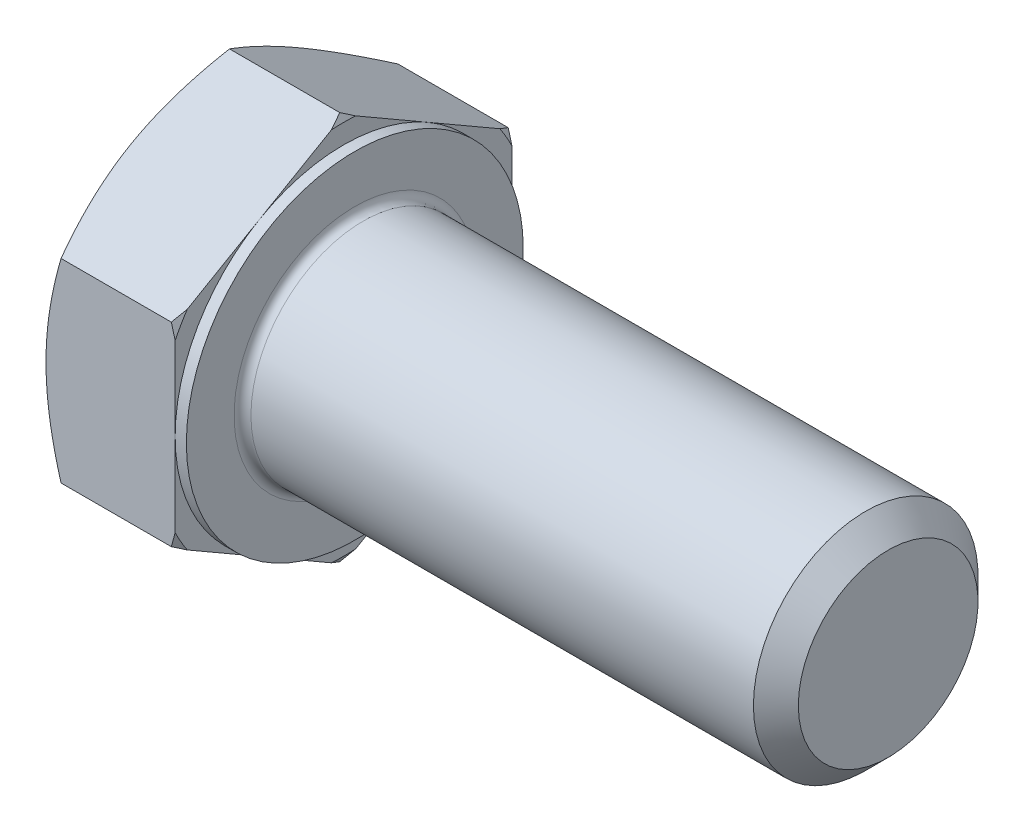
SolidWorks part; units mm, degrees
material "SAE2"
ref_plane "Front" through (0, 0, 0) normal (0, 0, 1) x (1, 0, 0)
ref_plane "Top" through (0, 0, 0) normal (0, 1, 0) x (1, 0, 0)
ref_plane "Right" through (0, 0, 0) normal (1, 0, 0) x (0, 0, -1)
sketch "Sketch1" plane through (0, 0, 0) normal (1, 0, 0) x (0, 0, -1)
  line L0 (12, 6.9282) -> (12, -6.9282)
  line L1 (-12, 6.9282) -> (-12, -6.9282)
  line L2 (12, -6.9282) -> (0, -13.8564)
  line L3 (0, -13.8564) -> (-12, -6.9282)
  line L4 (12, 6.9282) -> (0, 13.8564)
  line L5 (0, 13.8564) -> (-12, 6.9282)
  dimension "s" = 24
  dimension "D2" = 120
  dimension "D3" = 12
  dimension "D4" = 12
  dimension "D5" = 12
extrude "Base-Extrude" add sketch "Sketch1" along normal blind 10
sketch "Sketch2" plane through (0, 0, 0) normal (0, 0, 1) x (1, 0, 0)
  line L0 (0, 6.9282) -> (0, -6.9282) construction
  line L1 (0, 0) -> (48, 0)
  line L2 (0, 0) -> (0, 8)
  line L3 (0, 8) -> (27.8072, 8)
  line L4 (48, 0) -> (48, 6.268)
  line L5 (10, 13.8564) -> (10, 6.9282) construction
  line L7 (0, 0) -> (96.52, 0) construction
  line L8 (48, -6.268) -> (27.8072, -8) construction
  line L9 (0, -8) -> (27.8072, -8) construction
  line L10 (12, 15.24) -> (12, -1.27) construction
  line L11 (10, 15.24) -> (10, -1.27) construction
  line L12 (10, 6.9282) -> (10, -6.9282) construction
  line L13 (27.8072, 8) -> (48, 8)
  line L14 (48, 8) -> (48, 6.268)
  dimension "l" = 38
  dimension "m" = 16
  dimension "Minor_dia" = 12.536
  dimension "p" = 2
  dimension "h" = 38
revolve "Boss-Revolve1" add sketch "Sketch2" angle 360 about L7
cosmetic thread "Helix1" parameters "Thread_length"=36, "Thread_minor"=12.536
sketch "Sketch3" plane through (0, 0, 0) normal (0, 0, 1) x (1, 0, 0)
  line L0 (0, 12) -> (3.9585, 18.8564)
  line L1 (0, 13.8564) -> (0, 6.9282) construction
  line L2 (3.9585, 18.8564) -> (3.9585, 23.8564)
  line L3 (3.9585, 23.8564) -> (-10, 23.8564)
  line L4 (-10, 23.8564) -> (-10, 12)
  line L5 (-10, 12) -> (0, 12)
  line L6 (0, 0) -> (99.06, 0) construction
  line L7 (10, 13.8564) -> (0, 13.8564) construction
  dimension "D1" = 12
  dimension "D2" = 5
  dimension "D3" = 10
  dimension "D4" = 5
  dimension "Head_ch_ang" = 30
revolve "Cut-Revolve1" cut sketch "Sketch3" angle 360 about L6
sketch "Sketch5" plane through (0, 0, 0) normal (0, 0, 1) x (1, 0, 0)
  line L0 (10, 12) -> (6.0415, 18.8564)
  line L1 (10, 13.8564) -> (10, 6.9282) construction
  line L2 (6.0415, 18.8564) -> (6.0415, 23.8564)
  line L3 (6.0415, 23.8564) -> (16.0415, 23.8564)
  line L4 (16.0415, 23.8564) -> (16.0415, 12)
  line L5 (16.0415, 12) -> (10, 12)
  line L7 (10, 13.8564) -> (1.0718, 13.8564) construction
  line L8 (0, 0) -> (99.06, 0) construction
  line L9 (0, 0) -> (99.06, 0) construction
  dimension "D1" = 12
  dimension "D2" = 5
  dimension "D3" = 10
  dimension "Head_ch_ang" = 30
  dimension "D4" = 5
revolve "Cut-Revolve2" cut sketch "Sketch5" angle 360 about L8
sketch "Sketch4" plane through (0, 0, 0) normal (0, 0, 1) x (1, 0, 0)
  line L1 (10, 13.8564) -> (10, 6.9282) construction
  line L2 (10, 12) -> (9.2, 12)
  line L3 (10, 12) -> (10, 23.8564)
  line L4 (10, 23.8564) -> (9.2, 23.8564)
  line L5 (0, 0) -> (95.25, 0) construction
  line L6 (0, 0) -> (96.52, 0) construction
  line L7 (9.2, 12) -> (9.2, 23.8564)
  line L8 (8.9282, 13.8564) -> (1.0718, 13.8564) construction
  dimension "D1" = 24
  dimension "D2" = 10
  dimension "c" = 0.8
revolve "Cut-Revolve3" cut sketch "Sketch4" angle 360 about L5
chamfer "Chamfer" distance 1.6 angle 45 1 edges at (48, 0, 8)
fillet "Fillet" radius 0.6 1 edges at (10, 0, -8)
sketch "Sketch6" plane through (0, 0, 0) normal (0, 0, 1) x (1, 0, 0)
  line L0 (12, -6.268) -> (11, -8)
  line L1 (12, -6.268) -> (13, -8)
  line L2 (13, -8) -> (13, -10)
  line L3 (-3.175, 0) -> (5.1513, 0) construction
  line L5 (13, -10) -> (11, -10)
  line L6 (11, -10) -> (11, -8)
  dimension "Thread_minor" = 12.536
  dimension "Diameter" = 16
  dimension "Start" = 12
  dimension "SideAngle" = 60
  dimension "VeeAngle" = 60
  dimension "Overcut" = 20
revolve "Cut-Revolve4" [suppressed] cut sketch "Sketch6" angle 360 about L3
pattern_linear "LPattern1" [suppressed]
